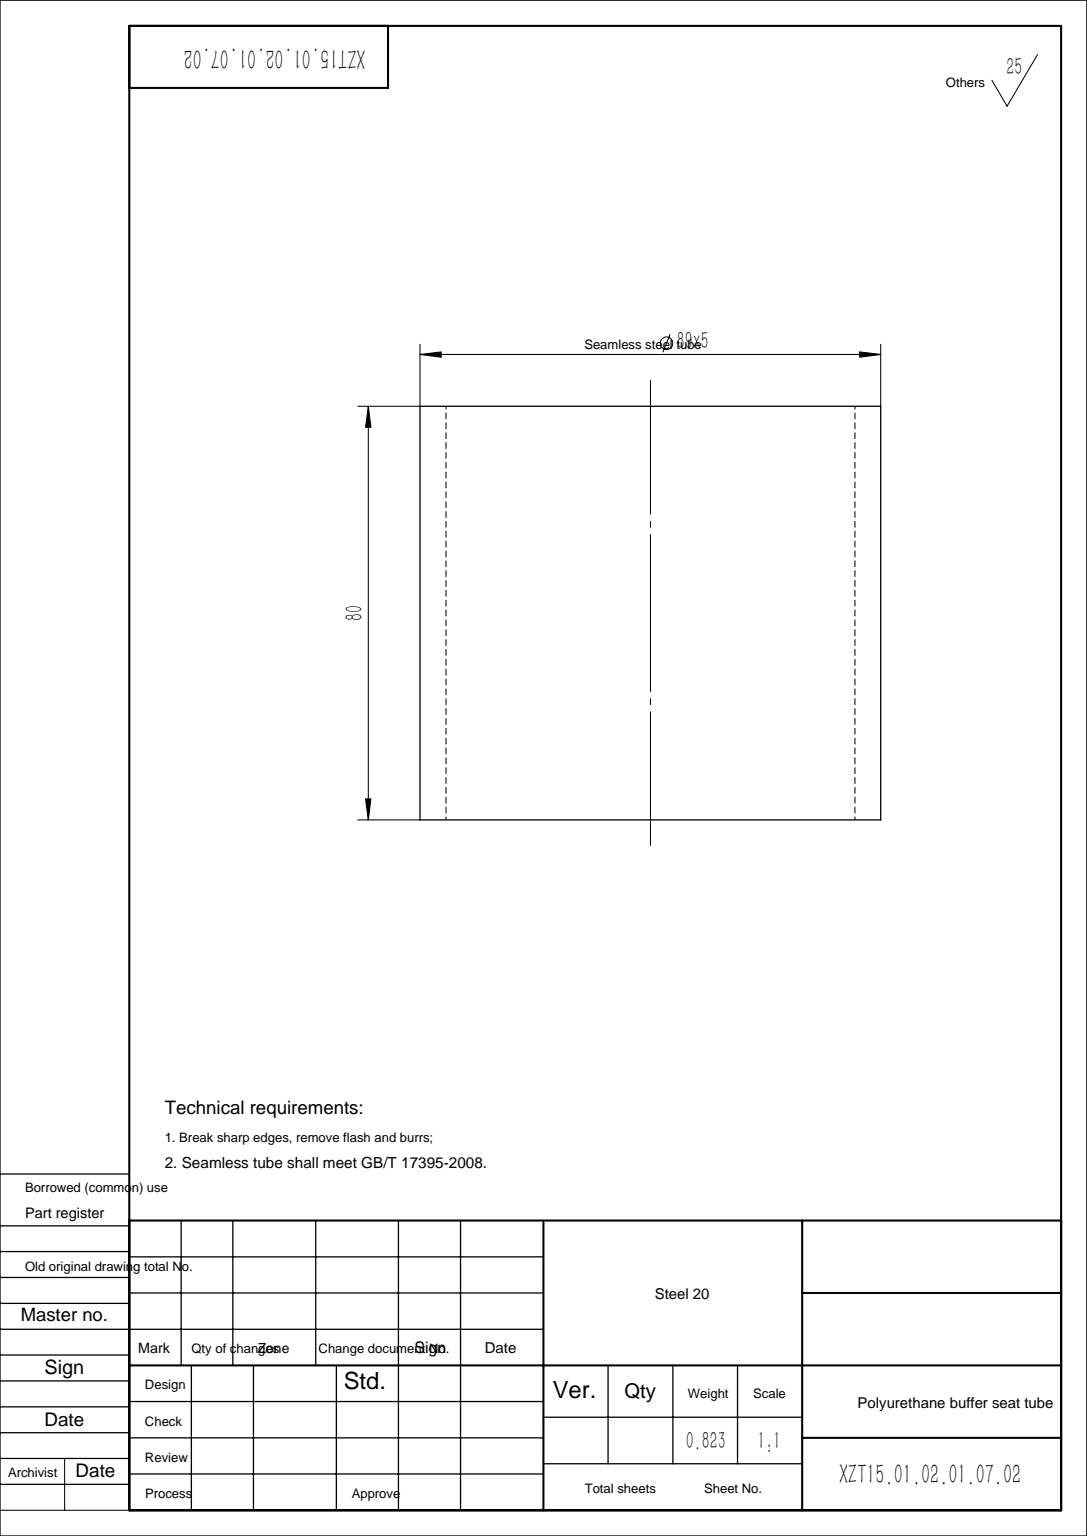
SolidWorks part; units mm, degrees
material "20 steel"
ref_plane "Front Plane" through (0, 0, 0) normal (0, 0, 1) x (1, 0, 0)
ref_plane "Top Plane" through (0, 0, 0) normal (0, 1, 0) x (1, 0, 0)
ref_plane "Right Plane" through (0, 0, 0) normal (1, 0, 0) x (0, 0, -1)
sketch "Sketch1" plane through (0, 0, 0) normal (0, 1, 0) x (1, 0, 0)
  circle A0 centre (0, 0) radius 44.5
  circle A1 centre (0, 0) radius 39.5
  dimension "D1" = 89
  dimension "D2" = 5
extrude "Boss-Extrude1" add sketch "Sketch1" along normal blind 80
